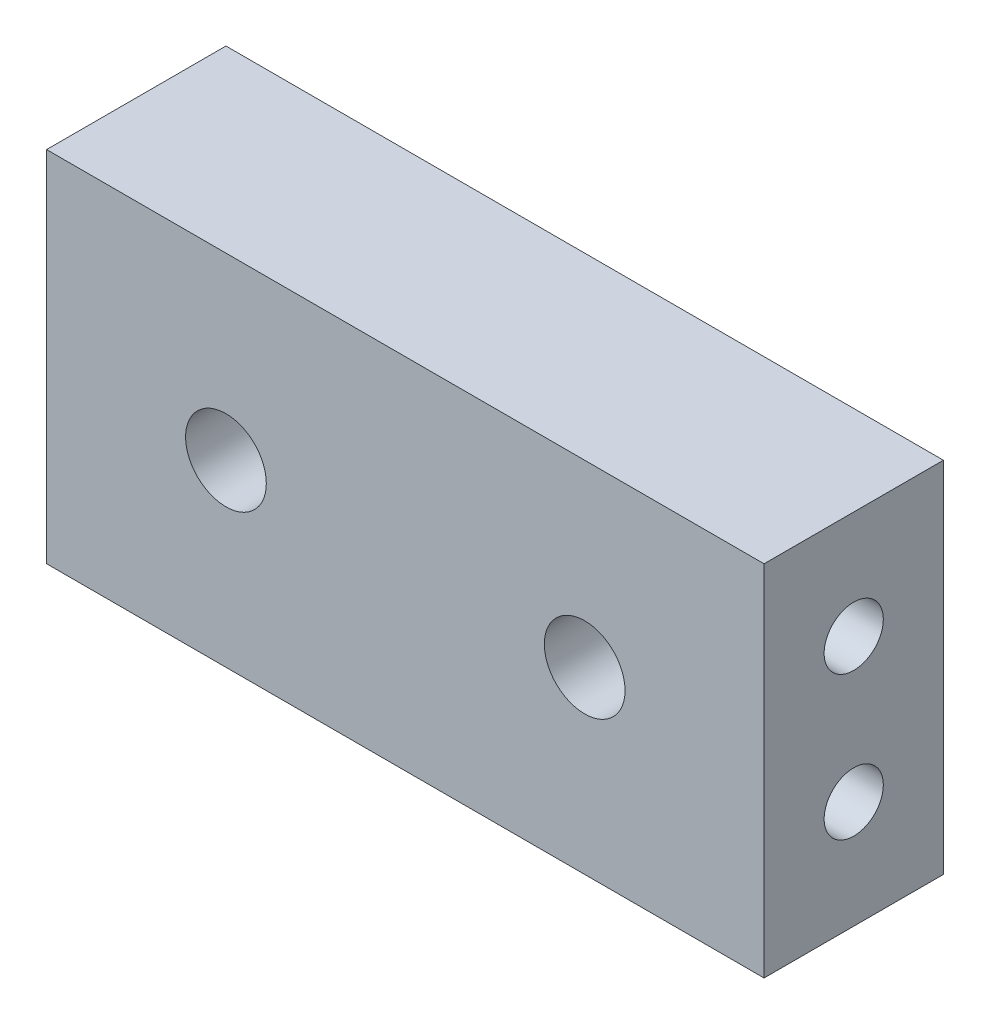
SolidWorks part; units mm, degrees
ref_plane "前视基准面" through (0, 0, 0) normal (0, 0, 1) x (1, 0, 0)
ref_plane "上视基准面" through (0, 0, 0) normal (0, 1, 0) x (1, 0, 0)
ref_plane "右视基准面" through (0, 0, 0) normal (1, 0, 0) x (0, 0, -1)
sketch "草图1" plane through (0, 0, 0) normal (0, 0, 1) x (1, 0, 0)
  line L1 (-19.3485, 10.1954) -> (20.6515, 10.1954)
  line L2 (-19.3485, 10.1954) -> (-19.3485, -9.8046)
  line L3 (-19.3485, -9.8046) -> (20.6515, -9.8046)
  line L4 (20.6515, 10.1954) -> (20.6515, -9.8046)
  circle A0 centre (-9.3485, 0.1954) radius 2.25
  circle A1 centre (10.6515, 0.1954) radius 2.25
  dimension "D3" = 4.5
  dimension "D6" = 4.5
  dimension "D1" = 40
  dimension "D2" = 20
  dimension "D4" = 10
  dimension "D5" = 10
  dimension "D7" = 10
  dimension "D8" = 10
extrude "凸台-拉伸1" add sketch "草图1" along normal blind 10
sketch "草图3" plane through (-19.3485, 0, 0) normal (-1, 0, 0) x (0, 0, 1)
  line L0 (10, 10.1954) -> (0, 10.1954) construction
  line L1 (10, 10.1954) -> (10, -9.8046) construction
  line L2 (10, -9.8046) -> (0, -9.8046) construction
  circle A0 centre (5, 4.1954) radius 1.65
  circle A1 centre (5, -3.8046) radius 1.65
  dimension "D5" = 3.3
  dimension "D6" = 3.3
  dimension "D1" = 6
  dimension "D2" = 5
  dimension "D3" = 6
  dimension "D4" = 5
extrude "切除-拉伸1" cut sketch "草图3" against normal blind 11.5
sketch "草图4" plane through (20.6515, 0, 0) normal (1, 0, 0) x (0, 0, -1)
  line L0 (0, -9.8046) -> (0, 10.1954) construction
  line L1 (-10, 10.1954) -> (0, 10.1954) construction
  line L2 (-10, -9.8046) -> (0, -9.8046) construction
  circle A0 centre (-5, 4.1954) radius 1.65
  circle A1 centre (-5, -3.8046) radius 1.65
  dimension "D5" = 3.3
  dimension "D6" = 3.3
  dimension "D1" = 5
  dimension "D2" = 6
  dimension "D3" = 5
  dimension "D4" = 6
extrude "切除-拉伸2" cut sketch "草图4" against normal blind 11.5
